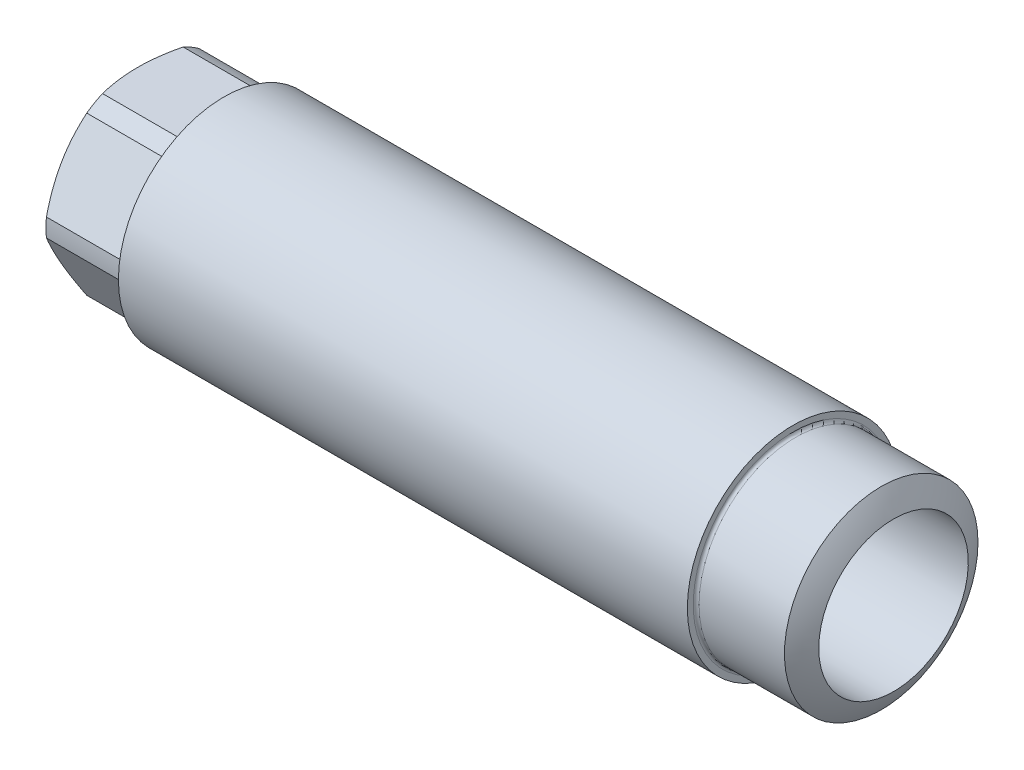
SolidWorks part; units mm, degrees
material "Plain Carbon Steel"
ref_plane "Front Plane" through (0, 0, 0) normal (0, 0, 1) x (1, 0, 0)
ref_plane "Top Plane" through (0, 0, 0) normal (0, 1, 0) x (1, 0, 0)
ref_plane "Right Plane" through (0, 0, 0) normal (1, 0, 0) x (0, 0, -1)
sketch "Sketch1" plane through (0, 0, 0) normal (1, 0, 0) x (0, 0, -1)
  circle A0 centre (0, 0) radius 18
  dimension "D1" = 36
extrude "Extrude1" add sketch "Sketch1" along normal blind 132
cosmetic thread "Cosmetic Thread1" parameters "D2"=33.8
sketch "Sketch2" plane through (0, 0, 0) normal (-1, 0, 0) x (0, 0, 1)
  circle A0 centre (0, 0) radius 12.75
  dimension "D1" = 25.5
extrude "Cut-Extrude1" cut sketch "Sketch2" against normal through all
sketch "Sketch3" plane through (0, 0, 0) normal (-1, 0, 0) x (0, 0, 1)
  circle A0 centre (0, 0) radius 16.5
  circle A2 centre (0, 0) radius 18 construction
  circle A3 centre (0, 0) radius 18
  dimension "D1" = 33
extrude "Cut-Extrude2" cut sketch "Sketch3" against normal blind 15
sketch "Sketch4" plane through (132, 0, 0) normal (1, 0, 0) x (0, 0, -1)
  circle A0 centre (0, 0) radius 16.5
  circle A2 centre (0, 0) radius 18 construction
  circle A3 centre (0, 0) radius 18
  dimension "D1" = 33
extrude "Cut-Extrude3" cut sketch "Sketch4" against normal blind 20
fillet "Fillet1" radius 0.5 2 edges at (15, 0, 16.5) (112, 0, -16.5)
sketch "Sketch5" plane through (0, 0, 0) normal (0, 0, 1) x (1, 0, 0)
  line L0 (132, -16.5) -> (132, 16.5) construction
  line L2 (119.0414, -42.2534) -> (137.0216, -42.2534)
  line L3 (137.0216, -42.2534) -> (137.0216, 0)
  line L5 (119.0414, -24.6899) -> (119.0414, -42.2534)
  line L6 (132, 0) -> (137.0216, 0)
  arc A0 (119.0414, -24.6899) -> (132, 0) centre (102, 0) ccw
  dimension "D1" = 60
  dimension "D6" = 42.2534
  dimension "D2" = 30
  dimension "D3" = 17.9802
  dimension "D4" = 17.5635
  dimension "D5" = 5.0216
revolve "Cut-Revolve1" cut sketch "Sketch5" angle 360 about axis through (132, 0, 0) along (-1, 0, 0)
sketch "Sketch6" plane through (0, 0, 0) normal (-1, 0, 0) x (0, 0, 1)
  line L0 (-8.6603, -15) -> (8.6603, -15)
  line L1 (8.6603, -15) -> (17.3205, 0)
  line L2 (17.3205, 0) -> (8.6603, 15)
  line L3 (8.6603, 15) -> (-8.6603, 15)
  line L4 (-8.6603, 15) -> (-17.3205, 0)
  line L5 (-17.3205, 0) -> (-8.6603, -15)
  circle A1 centre (0, 0) radius 25
  dimension "D6" = 50
  dimension "D1" = 15
  dimension "D2" = 120
  dimension "D3" = 120
  dimension "D4" = 30
  dimension "D5" = 8.6603
extrude "Cut-Extrude4" cut sketch "Sketch6" against normal blind 14
sketch "Sketch7" plane through (0, 0, 0) normal (0, 0, 1) x (1, 0, 0)
  line L0 (0, -14.5) -> (0, -24.5)
  line L1 (0, -24.5) -> (5.7735, -24.5)
  line L2 (5.7735, -24.5) -> (0, -14.5)
  dimension "D1" = 14.5
  dimension "D2" = 30
  dimension "D3" = 10
revolve "Cut-Revolve2" cut sketch "Sketch7" angle 360 about axis through (15, 0, 0) along (-1, 0, 0)
